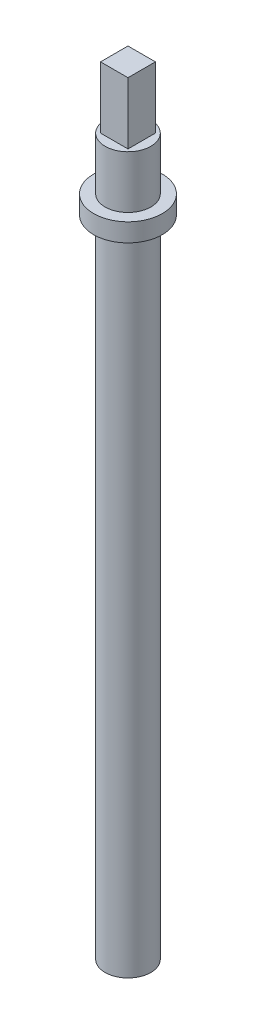
SolidWorks part; units mm, degrees
ref_plane "Front Plane" through (0, 0, 0) normal (0, 0, 1) x (1, 0, 0)
ref_plane "Top Plane" through (0, 0, 0) normal (0, 1, 0) x (1, 0, 0)
ref_plane "Right Plane" through (0, 0, 0) normal (1, 0, 0) x (0, 0, -1)
sketch "Sketch1" plane through (0, 0, 0) normal (0, 1, 0) x (1, 0, 0)
  circle A0 centre (0, 0) radius 10
  dimension "D1" = 20
extrude "Boss-Extrude1" add sketch "Sketch1" along normal blind 340
sketch "Sketch2" plane through (0, 340, 0) normal (0, 1, 0) x (1, 0, 0)
  line L5 (-6, 6) -> (6, 6)
  line L6 (-6, 6) -> (-6, -6)
  line L7 (-6, -6) -> (6, -6)
  line L8 (6, 6) -> (6, -6)
  line L9 (-6, 6) -> (6, -6) construction
  line L10 (-6, -6) -> (6, 6) construction
  point P0 (0, 0)
  dimension "D1" = 12
extrude "Cut-Extrude1" cut sketch "Sketch2" against normal blind 27 flip side to cut
ref_plane "Plane1" through (0, 282, 0) normal (0, 1, 0) x (1, 0, 0)
sketch "Sketch3" plane through (0, 282, 0) normal (0, 1, 0) x (1, 0, 0)
  circle A0 centre (0, 0) radius 15
  dimension "D1" = 30
extrude "Boss-Extrude2" add sketch "Sketch3" along normal blind 8
